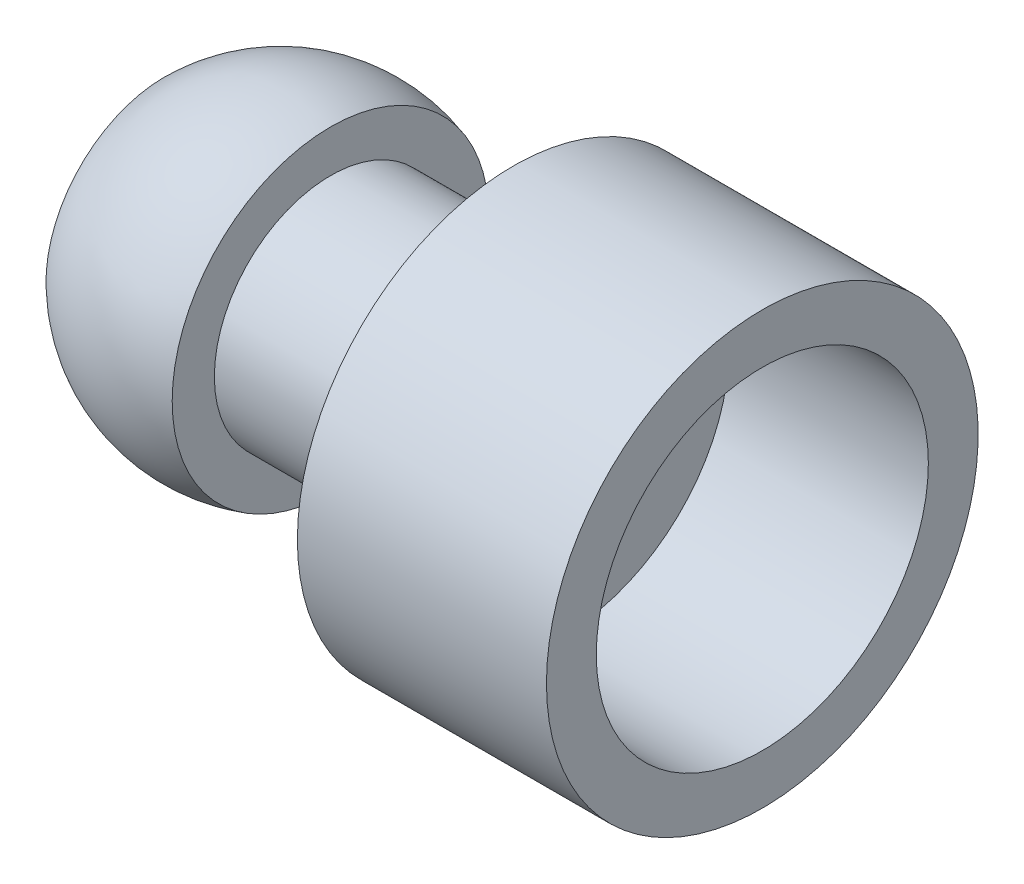
from build123d import *


with BuildPart() as part:
    # Sketch1 → Revolve1 (revolve)
    with BuildSketch(Plane(origin=(0, 0, 0), x_dir=(-1, 0, 0), z_dir=(0, 0, -1)), mode=Mode.PRIVATE) as revolve1_sk:
        with BuildLine():
            Line((21, 5), (23.886751346, 0))
            Line((23.886751346, 0), (36, 0))
            Line((36, 0), (36, 7.141428429))
            ThreePointArc((36, 7.141428429), (31.331857058, 9.724322221), (26, 9.539392014))
            Line((26, 9.539392014), (26, 7))
            Line((26, 7), (15, 7))
            Line((15, 7), (15, 13))
            Line((15, 13), (0, 13))
            Line((0, 13), (0, 10))
            Line((0, 10), (12, 10))
            Line((12, 10), (12, 5))
            Line((12, 5), (21, 5))
        make_face()
    revolve(revolve1_sk.sketch.rotate(Axis((0, 0, 0), (-1, 0, 0)), 270), axis=Axis((0, 0, 0), (-1, 0, 0)))


solid = part.part
